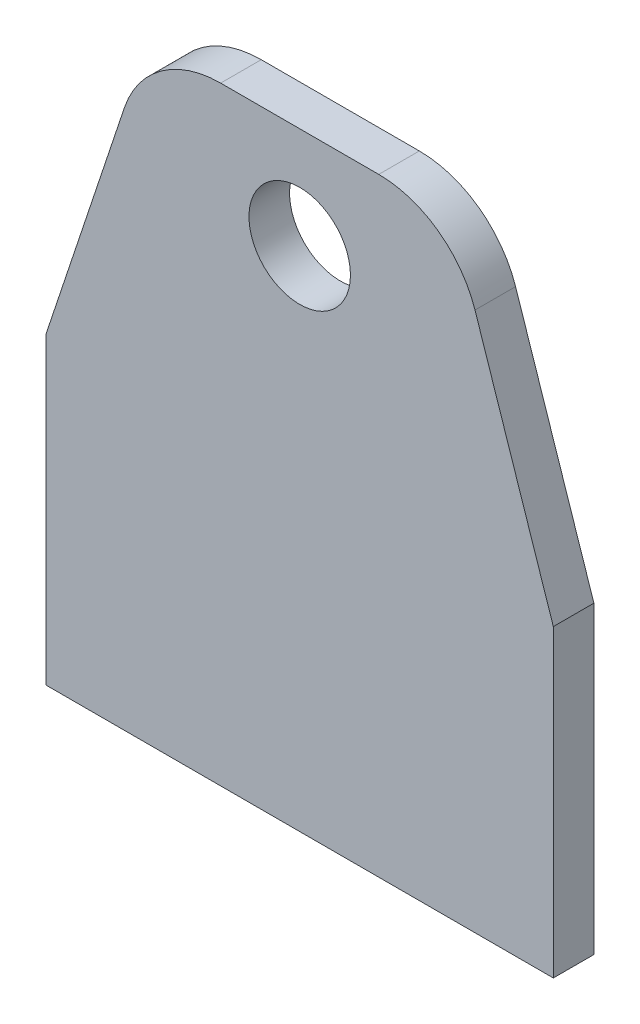
from build123d import *

# Parameters (mm, degrees)
SKETCH1_R           = 5
BOSS_EXTRUDE1_DEPTH = 4


with BuildPart() as part:
    # Sketch1 → Boss-Extrude1 (new body)
    with BuildSketch(Plane.XY):
        with BuildLine():
            Line((33.433153565, 28.077762704), (17.848337966, 28.077762704))
            ThreePointArc((17.848337966, 28.077762704), (12.001235119, 26.190184555), (8.361504986, 21.240040364))
            Line((8.361504986, 21.240040364), (0.640745765, -1.922237296))
            Line((0.640745765, -1.922237296), (0.640745765, -31.922237296))
            Line((0.640745765, -31.922237296), (50.640745765, -31.922237296))
            Line((50.640745765, -31.922237296), (50.640745765, -1.922237296))
            Line((50.640745765, -1.922237296), (42.919986545, 21.240040364))
            ThreePointArc((42.919986545, 21.240040364), (39.280256412, 26.190184555), (33.433153565, 28.077762704))
        make_face()
        with Locations((25.640745765, 18.077762704)):
            Circle(SKETCH1_R, mode=Mode.SUBTRACT)
    extrude(amount=BOSS_EXTRUDE1_DEPTH)


solid = part.part
